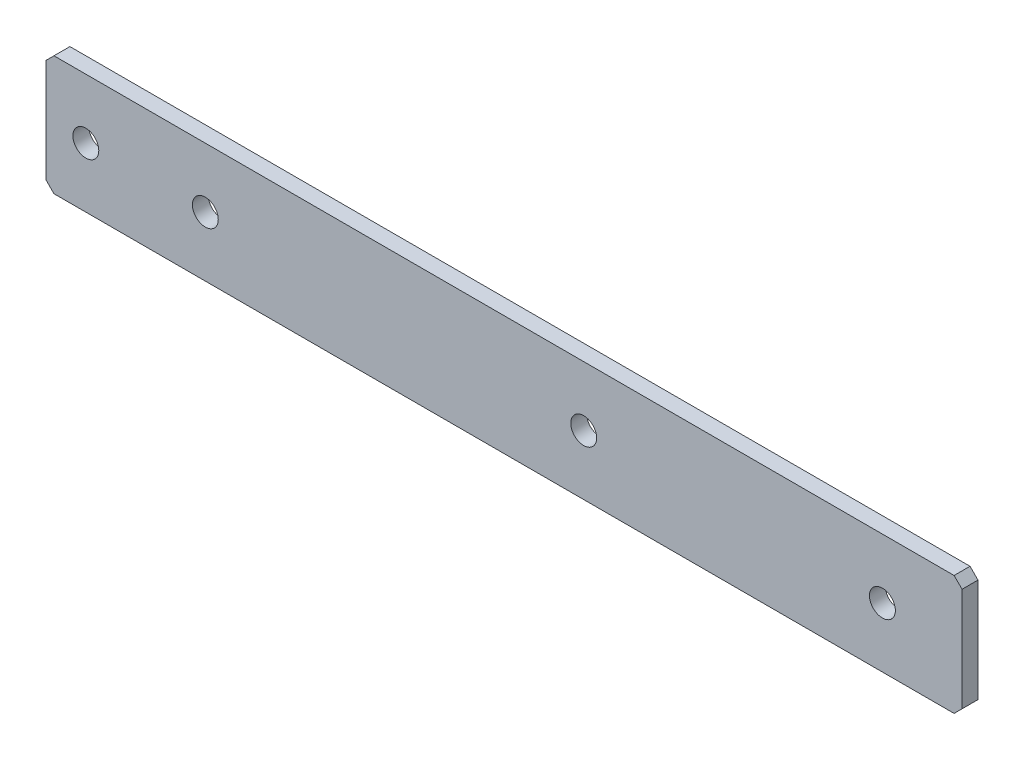
from build123d import *

# Parameters (mm, degrees)
SKETCH1_W           = 230
SKETCH1_H           = 30
SKETCH1_R           = 3.25
BOSS_EXTRUDE1_DEPTH = 4
CHAMFER1_SIZE       = 2


with BuildPart() as part:
    # Sketch1 → Boss-Extrude1 (new body)
    with BuildSketch(Plane.XY):
        Rectangle(SKETCH1_W, SKETCH1_H)
        with Locations((-105, 0)):
            Circle(SKETCH1_R, mode=Mode.SUBTRACT)
        with Locations((-75, 0)):
            Circle(SKETCH1_R, mode=Mode.SUBTRACT)
        with Locations((20, 0)):
            Circle(SKETCH1_R, mode=Mode.SUBTRACT)
        with Locations((95, 0)):
            Circle(SKETCH1_R, mode=Mode.SUBTRACT)
    extrude(amount=BOSS_EXTRUDE1_DEPTH)

    # Chamfer1
    chamfer1_edges = [part.edges().sort_by_distance(p)[0] for p in [
        (-115, 15, 2),
        (115, 15, 2),
        (115, -15, 2),
        (-115, -15, 2),
    ]]
    chamfer(chamfer1_edges, length=CHAMFER1_SIZE)


solid = part.part
